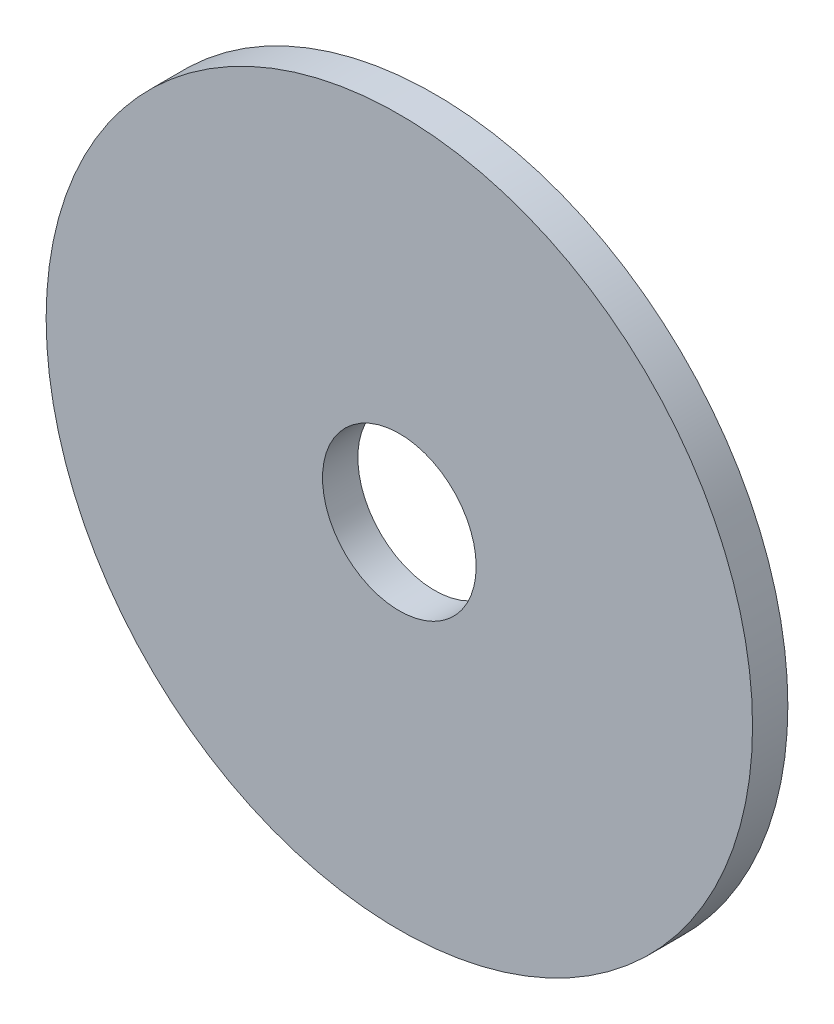
SolidWorks part; units mm, degrees
ref_plane "前视基准面" through (0, 0, 0) normal (0, 0, 1) x (1, 0, 0)
ref_plane "上视基准面" through (0, 0, 0) normal (0, 1, 0) x (1, 0, 0)
ref_plane "右视基准面" through (0, 0, 0) normal (1, 0, 0) x (0, 0, -1)
sketch "草图1" plane through (0, 0, 0) normal (0, 0, 1) x (1, 0, 0)
  circle A0 centre (0, 0) radius 100
  circle A1 centre (0, 0) radius 21.75
  dimension "D1" = 200
  dimension "D2" = 43.5
extrude "凸台-拉伸1" add sketch "草图1" along normal blind 10
